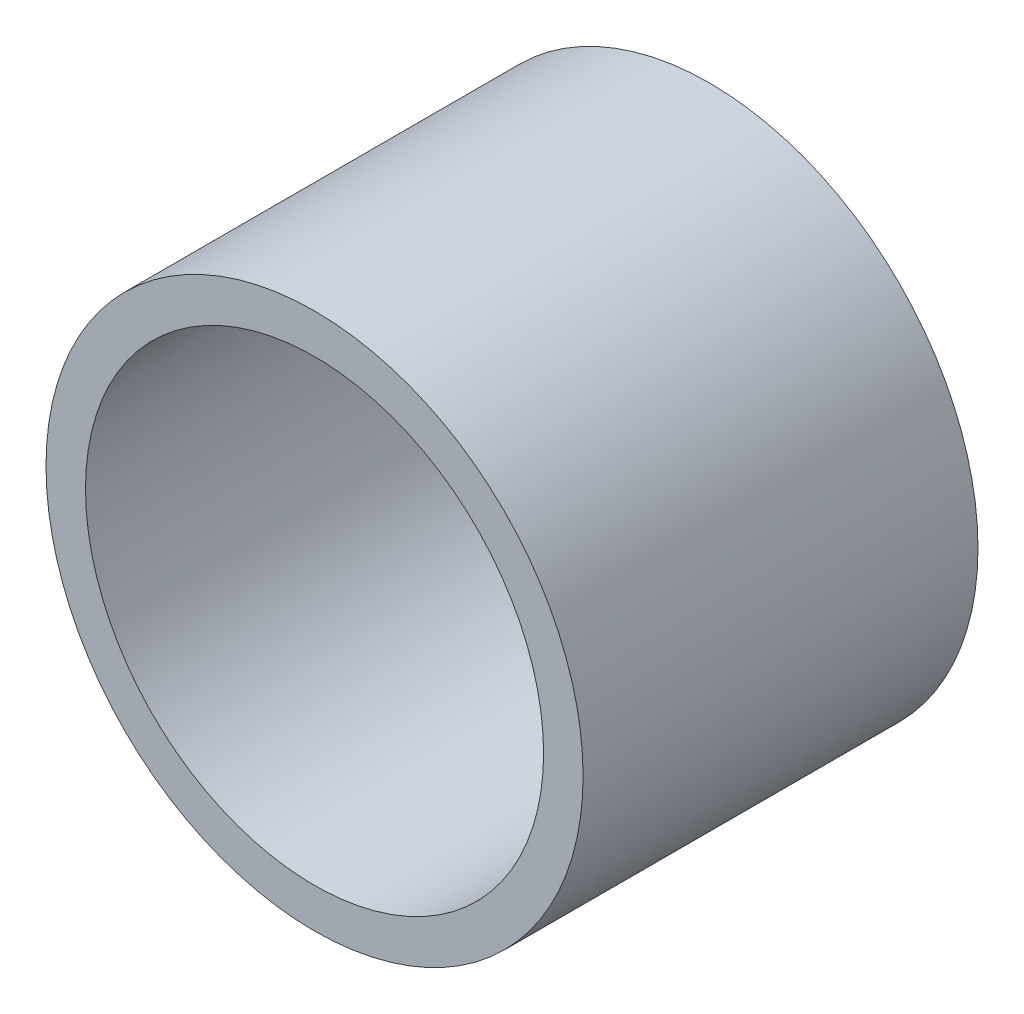
from build123d import *

# Parameters (mm, degrees)
SKETCH1_R           = 34
BOSS_EXTRUDE1_DEPTH = 50
SHELL1_T            = -5


with BuildPart() as part:
    # Sketch1 → Boss-Extrude1 (new body)
    with BuildSketch(Plane.XY):
        Circle(SKETCH1_R)
    extrude(amount=BOSS_EXTRUDE1_DEPTH)

    # Shell1
    shell1_openings = [part.faces().sort_by_distance(p)[0] for p in [
        (0, 0, 50),
    ]]
    offset(amount=SHELL1_T, openings=shell1_openings, kind=Kind.INTERSECTION)


solid = part.part
